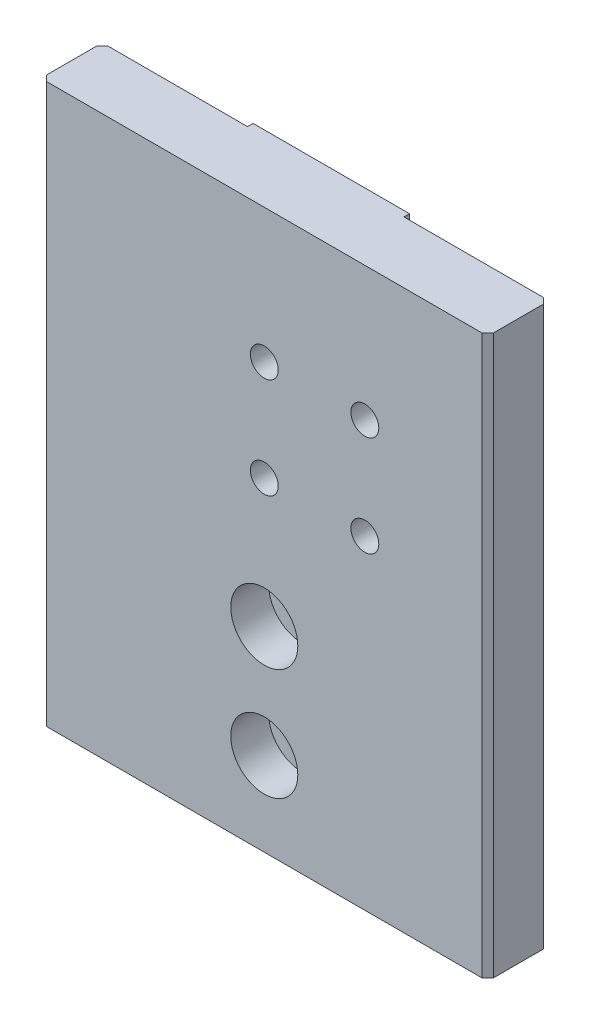
SolidWorks part; units mm, degrees
ref_plane "Front Plane" through (0, 0, 0) normal (0, 0, 1) x (1, 0, 0)
ref_plane "Top Plane" through (0, 0, 0) normal (0, 1, 0) x (1, 0, 0)
ref_plane "Right Plane" through (0, 0, 0) normal (1, 0, 0) x (0, 0, -1)
sketch "Sketch1" plane through (0, 0, 0) normal (0, 1, 0) x (1, 0, 0)
  line L0 (0, 0) -> (40, 0)
  line L1 (40, 0) -> (40, 5.5)
  line L2 (40, 5.5) -> (27, 5.5)
  line L3 (27, 5.5) -> (27, 6)
  line L4 (27, 6) -> (13, 6)
  line L5 (13, 6) -> (13, 5.5)
  line L6 (13, 5.5) -> (0, 5.5)
  line L7 (0, 5.5) -> (0, 0)
  line L8 (20, 0) -> (20, 11.6331) construction
  dimension "D1" = 40
  dimension "D2" = 5.5
  dimension "D3" = 0.5
  dimension "D4" = 14
extrude "Boss-Extrude1" add sketch "Sketch1" along normal mid plane 50
chamfer "Chamfer1" distance 0.5 angle 45 4 edges at (40, 0, -5.5) (40, 0, 0) (0, 0, 0) (0, 0, -5.5)
hole_wizard "Hole Size per Socket Head Cap Screw Type1" positions "Sketch3" profile "Sketch2" counterbore size "M3" standard "GB" end condition through all
sketch "Sketch3" plane through (0, 0, 0) normal (0, 0, 1) x (1, 0, 0)
  line L0 (20, 25) -> (20, -26.8902) construction
  line L1 (0.5, 25) -> (39.5, 25) construction
  line L4 (0.5, -25) -> (39.5, -25) construction
  point P1 (20, -7.5)
  point P16 (20, -17.5)
  dimension "D1" = 7.5
  dimension "D2" = 10
sketch "Sketch2" plane through (20, -7.5, 0) normal (1, 0, 0) x (0, -1, 0)
  line L0 (0, 0) -> (0, 6)
  line L1 (0, 6) -> (1.7, 6)
  line L3 (1.7, 6) -> (1.7, 3.4)
  line L4 (1.7, 3.4) -> (3, 3.4)
  line L5 (3, 3.4) -> (3, 0)
  line L7 (3, 0) -> (0, 0)
  line L11 (0, -6.35) -> (0, 107.95) construction
  dimension "通孔孔直径" = 3.4
  dimension "通孔孔深度" = 6
  dimension "柱形沉头孔直径" = 6
  dimension "柱形沉头孔深度" = 3.4
hole_wizard "M3 Tapped Hole1" positions "Sketch5" profile "Sketch4" tap size "M3" standard "GB"
sketch "Sketch5" plane through (0, 0, 0) normal (0, 0, 1) x (1, 0, 0)
  line L3 (20, 25) -> (20, -36.0107) construction
  line L4 (0.5, 25) -> (39.5, 25) construction
  line L5 (40, 25) -> (40, -25) construction
  point P0 (20, 13)
  point P1 (29, 13)
  point P14 (20, 4)
  point P16 (29, 4)
  dimension "D1" = 9
  dimension "D2" = 12
  dimension "D3" = 9
  dimension "D4" = 11
sketch "Sketch4" plane through (20, 13, 0) normal (1, 0, 0) x (0, -1, 0)
  line L0 (0, 0) -> (0, 8.2511)
  line L1 (0, 8.2511) -> (1.25, 7.5)
  line L2 (1.25, 7.5) -> (1.25, 0)
  line L5 (1.25, 0) -> (0, 0)
  line L10 (0, 8.2511) -> (-1.25, 7.5) construction
  line L11 (0, -6.35) -> (0, 107.95) construction
  dimension "螺纹孔钻头直径" = 2.5
  dimension "螺纹孔钻头深度" = 7.5
  dimension "导头角度" = 118
cosmetic thread "Cosmetic Thread1" parameters "D1"=5.5, "D2"=3
cosmetic thread "Cosmetic Thread2" parameters "D1"=5.5, "D2"=3
cosmetic thread "Cosmetic Thread3" parameters "D1"=5.5, "D2"=3
cosmetic thread "Cosmetic Thread4" parameters "D1"=5.5, "D2"=3
